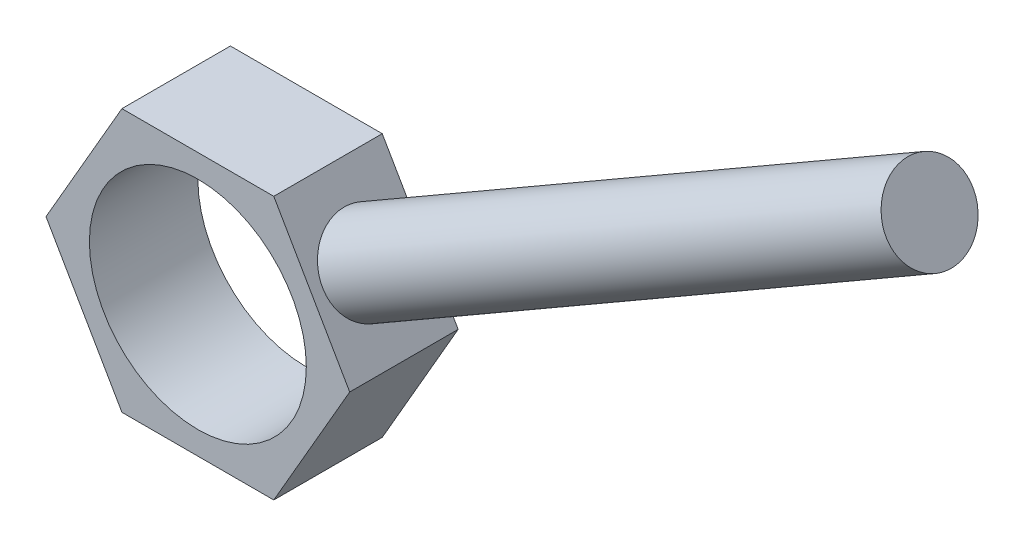
SolidWorks part; units mm, degrees
ref_plane "Front Plane" through (0, 0, 0) normal (0, 0, 1) x (1, 0, 0)
ref_plane "Top Plane" through (0, 0, 0) normal (0, 1, 0) x (1, 0, 0)
ref_plane "Right Plane" through (0, 0, 0) normal (1, 0, 0) x (0, 0, -1)
sketch "Sketch1" plane through (0, 0, 0) normal (0, 0, 1) x (1, 0, 0)
  line L1 (-3.5, 6.0622) -> (-7, 0)
  line L2 (-7, 0) -> (-3.5, -6.0622)
  line L3 (-3.5, -6.0622) -> (3.5, -6.0622)
  line L4 (3.5, -6.0622) -> (7, 0)
  line L5 (7, 0) -> (3.5, 6.0622)
  line L6 (3.5, 6.0622) -> (-3.5, 6.0622)
  circle A0 centre (0, 0) radius 5
  circle A1 centre (0, 0) radius 6.0622 construction
  dimension "D1" = 10
  dimension "D2" = 14
extrude "Boss-Extrude1" add sketch "Sketch1" along normal blind 5
sketch "Sketch2" plane through (5.25, 3.0311, 0) normal (0.866, 0.5, 0) x (0, 0, -1)
  circle A0 centre (-2.5, 0) radius 2
  dimension "D1" = 4
extrude "Boss-Extrude2" add sketch "Sketch2" along normal blind 30
